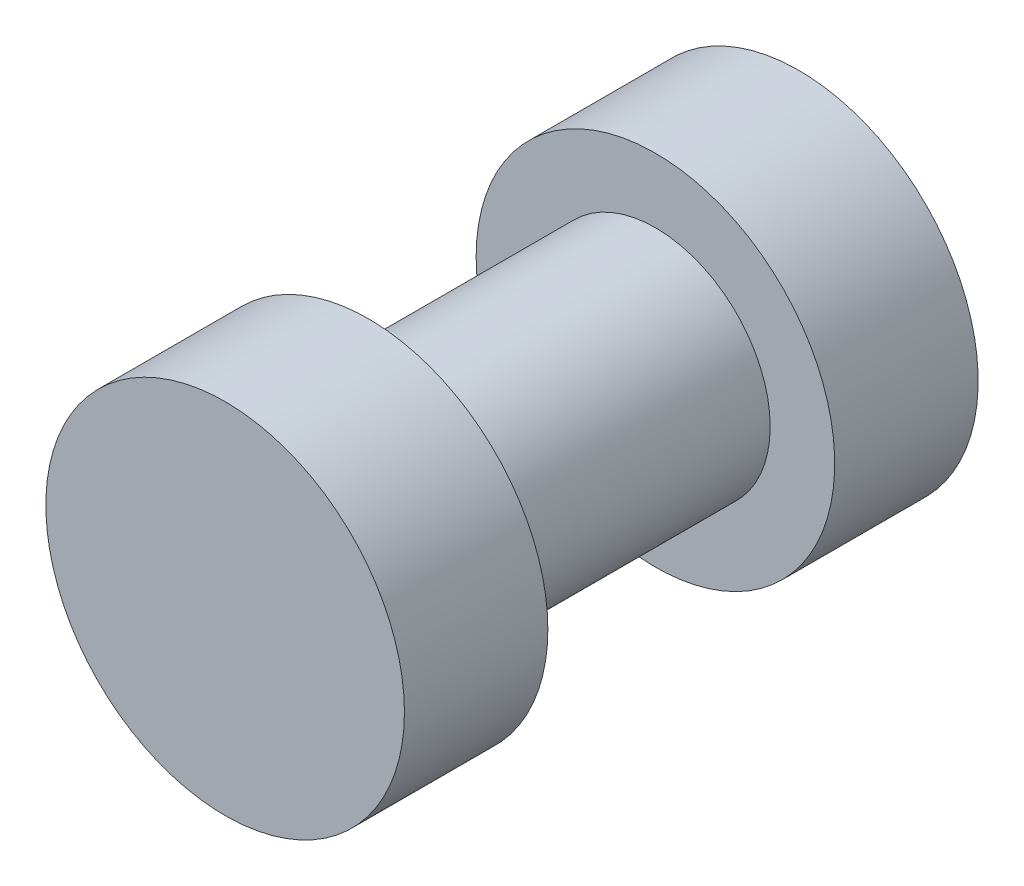
from build123d import *

# Parameters (mm, degrees)
SKETCH1_R           = 8
BOSS_EXTRUDE1_DEPTH = 20
SKETCH2_R           = 12.5
BOSS_EXTRUDE2_DEPTH = 10
BOSS_EXTRUDE3_START = 10
SKETCH3_R           = 12.5
BOSS_EXTRUDE3_DEPTH = 10


with BuildPart() as part:
    # Sketch1 → Boss-Extrude1 (new body)
    with BuildSketch(Plane.XY):
        Circle(SKETCH1_R)
    extrude(amount=BOSS_EXTRUDE1_DEPTH)

    # Sketch2 → Boss-Extrude2 (add)
    with BuildSketch(Plane.XY.offset(20)):
        Circle(SKETCH2_R)
    extrude(amount=BOSS_EXTRUDE2_DEPTH)

    # Sketch3 → Boss-Extrude3 (add)
    with BuildSketch(Plane(origin=(0, 0, 0), x_dir=(-1, 0, 0), z_dir=(0, 0, -1)).offset(BOSS_EXTRUDE3_START)):
        with Locations(Location((0, 0, 0), (0, 0, 180))):
            Circle(SKETCH3_R)
    extrude(amount=-BOSS_EXTRUDE3_DEPTH)


solid = part.part
